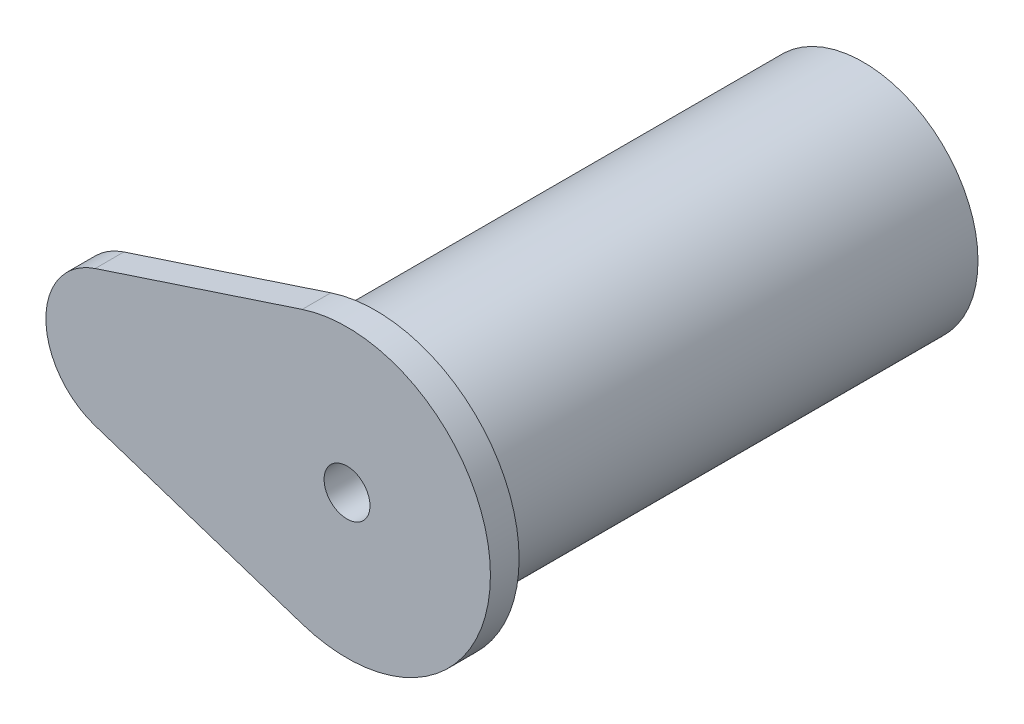
SolidWorks part; units mm, degrees
ref_plane "前视基准面" through (0, 0, 0) normal (0, 0, 1) x (1, 0, 0)
ref_plane "上视基准面" through (0, 0, 0) normal (0, 1, 0) x (1, 0, 0)
ref_plane "右视基准面" through (0, 0, 0) normal (1, 0, 0) x (0, 0, -1)
sketch "草图1" plane through (0, 0, 0) normal (0, 0, 1) x (1, 0, 0)
  circle A0 centre (0, 0) radius 20
extrude "凸台-拉伸1" add sketch "草图1" along normal blind 90
sketch "草图2" plane through (0, 0, 90) normal (0, 0, 1) x (1, 0, 0)
  line L1 (-43.9062, 11.874) -> (-7.8125, 23.7479)
  line L2 (-7.8125, -23.7479) -> (-43.9062, -11.874)
  arc A0 (-7.8125, -23.7479) -> (-7.8125, 23.7479) centre (0, 0) ccw
  arc A1 (-43.9062, 11.874) -> (-43.9062, -11.874) centre (-40, 0) ccw
extrude "凸台-拉伸2" add sketch "草图2" against normal blind 5
sketch "草图3" plane through (0, 0, 90) normal (0, 0, 1) x (1, 0, 0)
  circle A0 centre (0, 0) radius 4
extrude "切除-拉伸1" cut sketch "草图3" against normal blind 60
cosmetic thread "装饰螺纹线2" parameters "D1"=10, "D2"=9
sketch "草图4" plane through (0, 0, 0) normal (0, 1, 0) x (1, 0, 0)
  line L0 (0, 0) -> (0, -85)
  line L1 (25, -85) -> (-7.8125, -85) construction
  circle A0 centre (0, -42.5) radius 4
extrude "切除-拉伸2" cut sketch "草图4" against normal blind 20 contours L0 A0 | L0 A0
